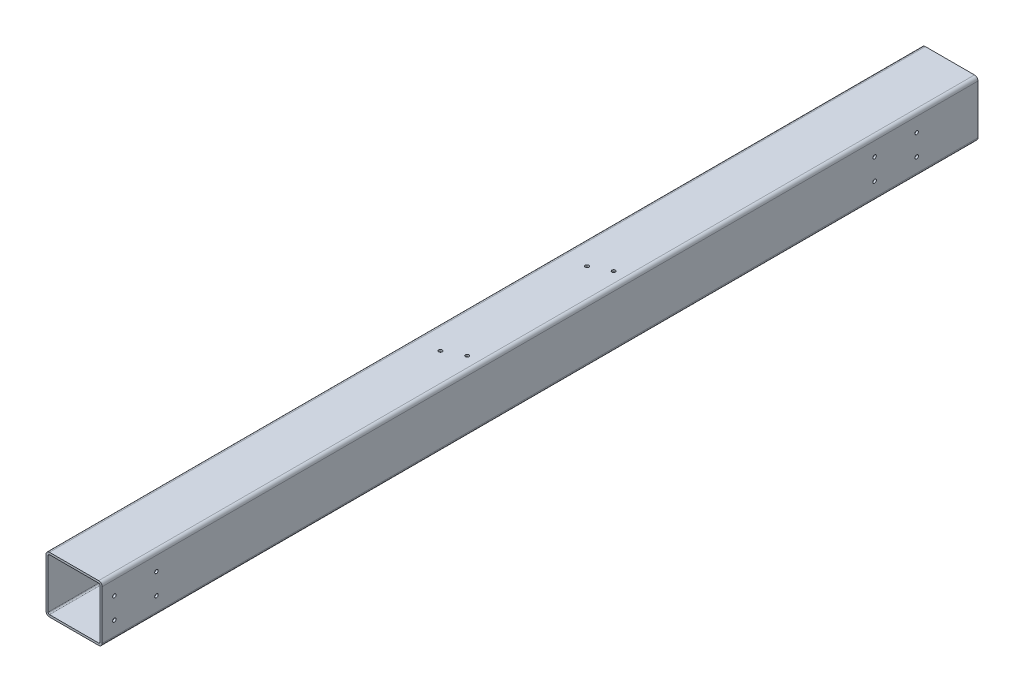
from build123d import *

# Parameters (mm, degrees)
SKETCH_1_W             = 80
SKETCH_1_H             = 80
EXTRUDE_1_DEPTH        = 1249
FILLET_1_R             = 5
SHELL_1_T              = -3
HOLE_WIZARD_M6_1_D     = 5
HOLE_WIZARD_M6_1_DEPTH = 15
HOLE_WIZARD_M6_1_TIP   = 1.502151548
HOLE_WIZARD_M6_2_D     = 5
HOLE_WIZARD_M6_2_DEPTH = 15
HOLE_WIZARD_M6_2_TIP   = 1.502151548
HOLE_WIZARD_M6_3_D     = 5
HOLE_WIZARD_M6_3_DEPTH = 15
HOLE_WIZARD_M6_3_TIP   = 1.502151548


with BuildPart() as part:
    # 草图1 → 凸台-拉伸1 (new body)
    with BuildSketch(Plane.XY):
        Rectangle(SKETCH_1_W, SKETCH_1_H)
    extrude(amount=EXTRUDE_1_DEPTH)

    # 圆角1
    fillet_1_edges = [part.edges().sort_by_distance(p)[0] for p in [
        (-40, 40, 624.5),
        (40, 40, 624.5),
        (40, -40, 624.5),
        (-40, -40, 624.5),
    ]]
    fillet(fillet_1_edges, radius=FILLET_1_R)

    # 抽壳1
    shell_1_openings = [part.faces().sort_by_distance(p)[0] for p in [
        (0, 0, 1249),
        (0, 0, 0),
    ]]
    offset(amount=SHELL_1_T, openings=shell_1_openings, kind=Kind.INTERSECTION)

    # M6 螺纹孔1
    with Locations(Plane(origin=(40, 0, 0), x_dir=(0, 0, -1), z_dir=(1, 0, 0))):
        with Locations((-147.5, 15), (-87.5, 15), (-87.5, -15), (-147.5, -15), (-1171.5, 15), (-1171.5, -15), (-1231.5, -15), (-1231.5, 15)):
            Hole(HOLE_WIZARD_M6_1_D / 2, depth=HOLE_WIZARD_M6_1_DEPTH)
            with Locations((0, 0, -(HOLE_WIZARD_M6_1_DEPTH + HOLE_WIZARD_M6_1_TIP / 2))):  # 118° drill point
                Cone(0, HOLE_WIZARD_M6_1_D / 2, HOLE_WIZARD_M6_1_TIP, mode=Mode.SUBTRACT)

    # M6 螺纹孔2
    with Locations(Plane(origin=(0, -40, 0), x_dir=(-1, 0, 0), z_dir=(0, -1, 0))):
        with Locations((-20, -749.5), (5, -736.5), (-20, -540.5), (5, -527.5)):
            Hole(HOLE_WIZARD_M6_2_D / 2, depth=HOLE_WIZARD_M6_2_DEPTH)
            with Locations((0, 0, -(HOLE_WIZARD_M6_2_DEPTH + HOLE_WIZARD_M6_2_TIP / 2))):  # 118° drill point
                Cone(0, HOLE_WIZARD_M6_2_D / 2, HOLE_WIZARD_M6_2_TIP, mode=Mode.SUBTRACT)

    # M6 螺纹孔3
    with Locations(Plane(origin=(0, 40, 0), x_dir=(1, 0, 0), z_dir=(0, 1, 0))):
        with Locations((-5, -721.5), (20, -708.5), (20, -499.5), (-5, -512.5)):
            Hole(HOLE_WIZARD_M6_3_D / 2, depth=HOLE_WIZARD_M6_3_DEPTH)
            with Locations((0, 0, -(HOLE_WIZARD_M6_3_DEPTH + HOLE_WIZARD_M6_3_TIP / 2))):  # 118° drill point
                Cone(0, HOLE_WIZARD_M6_3_D / 2, HOLE_WIZARD_M6_3_TIP, mode=Mode.SUBTRACT)


solid = part.part
